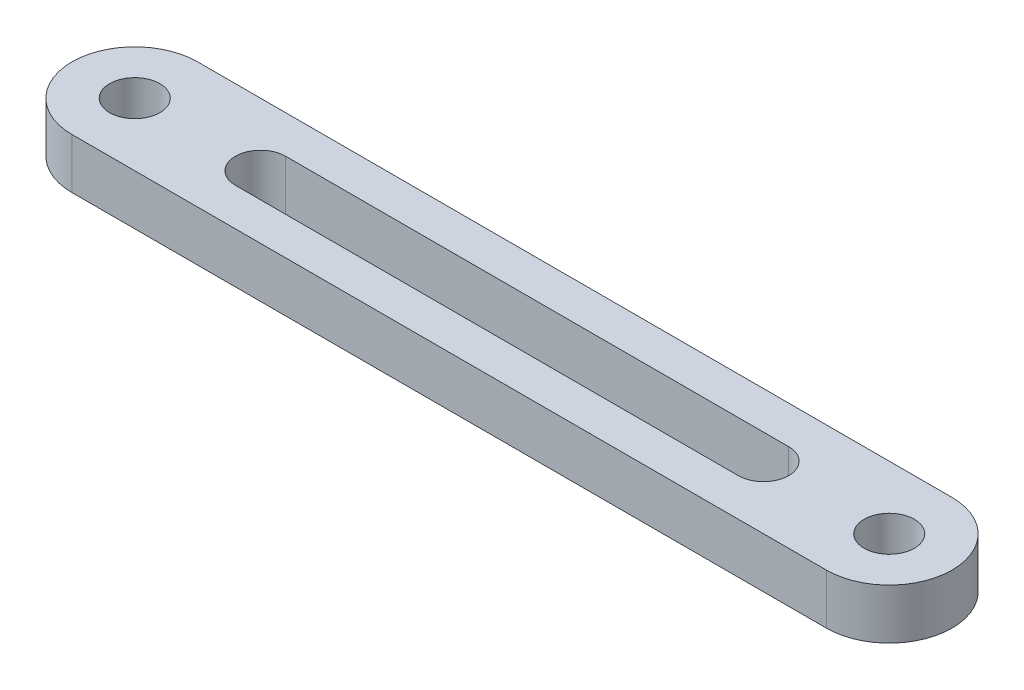
SolidWorks part; units mm, degrees
ref_plane "Front Plane" through (0, 0, 0) normal (0, 0, 1) x (1, 0, 0)
ref_plane "Top Plane" through (0, 0, 0) normal (0, 1, 0) x (1, 0, 0)
ref_plane "Right Plane" through (0, 0, 0) normal (1, 0, 0) x (0, 0, -1)
sketch "Sketch1" plane through (0, 0, 0) normal (0, 1, 0) x (1, 0, 0)
  line L0 (0, 12.5) -> (150, 12.5)
  line L1 (0, -12.5) -> (150, -12.5)
  circle A0 centre (0, 0) radius 5
  arc A1 (0, 12.5) -> (0, -12.5) centre (0, 0) ccw
  circle A2 centre (150, 0) radius 5
  arc A3 (150, -12.5) -> (150, 12.5) centre (150, 0) ccw
  dimension "D1" = 10
  dimension "D2" = 25
  dimension "D3" = 150
extrude "Boss-Extrude1" add sketch "Sketch1" along normal mid plane 10
sketch "Sketch2" plane through (0, 5, 0) normal (0, 1, 0) x (1, 0, 0)
  line L0 (25, 0) -> (125, 0) construction
  line L1 (25, 5) -> (125, 5)
  line L2 (25, -5) -> (125, -5)
  line L3 (75, 12.5) -> (75, 30.5851) construction
  line L4 (150, 12.5) -> (0, 12.5) construction
  arc A0 (25, 5) -> (25, -5) centre (25, 0) ccw
  arc A1 (125, -5) -> (125, 5) centre (125, 0) ccw
  point P3 (75, 0)
  dimension "D2" = 5
  dimension "D1" = 100
extrude "Cut-Extrude1" cut sketch "Sketch2" against normal blind 10
